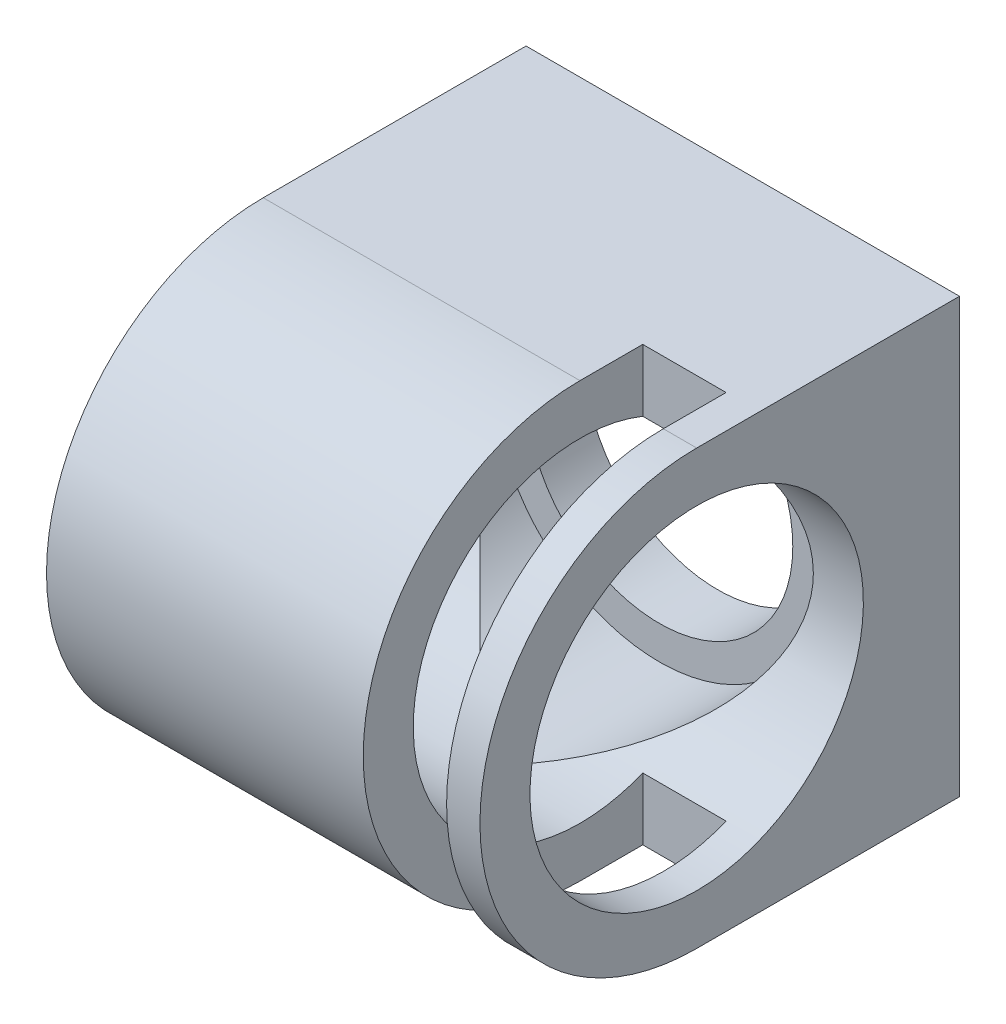
SolidWorks part; units mm, degrees
ref_plane "Front Plane" through (0, 0, 0) normal (0, 0, 1) x (1, 0, 0)
ref_plane "Top Plane" through (0, 0, 0) normal (0, 1, 0) x (1, 0, 0)
ref_plane "Right Plane" through (0, 0, 0) normal (1, 0, 0) x (0, 0, -1)
other "Configuration Table"
sketch "Sketch3" plane through (0, 0, 0) normal (0, 0, 1) x (1, 0, 0)
  line L0 (46.3215, 0) -> (-46.3215, 0) construction
  line L1 (0, -51.6969) -> (0, 51.6969) construction
  line L2 (-26, 26) -> (-26, -26)
  line L3 (-26, -26) -> (26, -26)
  line L4 (26, -26) -> (26, 26)
  line L5 (26, 26) -> (-26, 26)
  point P4 (0, 0)
  point P8 (0, 0)
  dimension "D1" = 52
  dimension "D2" = 52
extrude "Boss-Extrude1" add sketch "Sketch3" along normal blind 10
sketch "Sketch4" plane through (0, 0, 0) normal (0, 0, -1) x (-1, 0, 0)
  line L0 (0, -38.5407) -> (0, 38.5407) construction
  line L1 (-48.5266, 0) -> (48.5266, 0) construction
  circle A0 centre (-21, 21) radius 2
  circle A1 centre (21, 21) radius 2
  circle A2 centre (21, -21) radius 2
  circle A3 centre (-21, -21) radius 2
  point P6 (0, 0)
  point P10 (0, 0)
  dimension "D1" = 4
  dimension "D2" = 21
  dimension "D3" = 21
extrude "Cut-Extrude1" cut sketch "Sketch4" against normal blind 10
sketch "Sketch5" plane through (0, 0, 0) normal (0, 0, -1) x (-1, 0, 0)
  circle A0 centre (0, 0) radius 25
  dimension "D1" = 50
extrude "Cut-Extrude2" cut sketch "Sketch5" against normal blind 3
sketch "Sketch6" plane through (0, 0, 3) normal (0, 0, -1) x (-1, 0, 0)
  circle A0 centre (0, 0) radius 16
  dimension "D1" = 32
extrude "Cut-Extrude3" cut sketch "Sketch6" against normal through all
sketch "Sketch8" plane through (-26, 0, 0) normal (-1, 0, 0) x (0, 0, 1)
  line L0 (10, 26) -> (31.5315, 26)
  line L1 (31.5315, 26) -> (31.5315, -26)
  line L2 (10, -26) -> (31.5315, -26)
  line L3 (10, 26) -> (10, -26) construction
  line L4 (10, 26) -> (10, -26)
  dimension "D1" = 21.5315
extrude "Boss-Extrude2" add sketch "Sketch8" against normal blind 52
sketch "Sketch9" plane through (0, 0, 31.5315) normal (0, 0, 1) x (1, 0, 0)
  circle A0 centre (0, 0) radius 20
  dimension "D1" = 40
extrude "Cut-Extrude4" cut sketch "Sketch9" against normal blind 21.5315
sketch "Sketch10" plane through (-26, 0, 0) normal (-1, 0, 0) x (0, 0, 1)
  line L0 (31.5315, -26) -> (31.5315, 26) construction
  line L1 (31.5315, 26) -> (31.5315, -26)
  arc A0 (31.5315, -26) -> (31.5315, 26) centre (31.5315, 0) ccw
extrude "Boss-Extrude3" add sketch "Sketch10" against normal blind 52
sketch "Sketch11" plane through (-26, 0, 0) normal (-1, 0, 0) x (0, 0, 1)
  circle A0 centre (31.5315, 0) radius 20
  dimension "D1" = 40
extrude "Cut-Extrude5" cut sketch "Sketch11" against normal blind 52
ref_plane "Plane1" through (22, 0, 0) normal (1, 0, 0) x (0, 0, -1)
sketch "Sketch12" plane through (22, 0, 0) normal (1, 0, 0) x (0, 0, -1)
  line L0 (-68.3774, 0) -> (-37.4866, 0) construction
  line L1 (0, -26) -> (0, 26) construction
  line L2 (-58.659, 30) -> (-24, 30)
  line L3 (-58.659, 30) -> (-58.659, -30)
  line L4 (-58.659, -30) -> (-24, -30)
  line L5 (-24, 30) -> (-24, -30)
  dimension "D1" = 30
  dimension "D2" = 24
extrude "Cut-Extrude6" cut sketch "Sketch12" against normal blind 10
